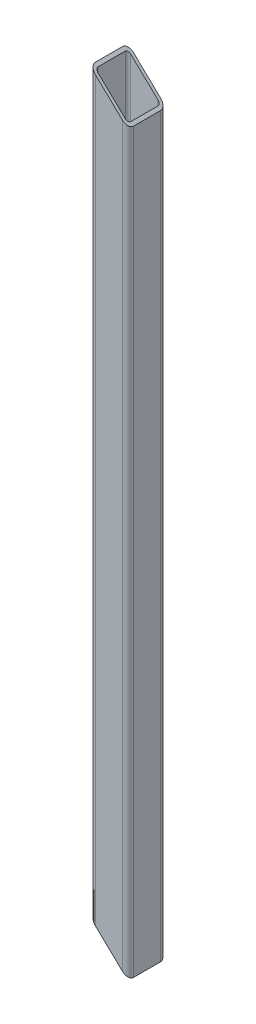
from build123d import *

# Parameters (mm, degrees)
FEATURE_19_WELDMEMBERFEAT_4_MORE_IN_5_DEPTH = 1420.5
CUT_EXTRUDE1_DEPTH                          = 1423.654297431
CUT_EXTRUDE1_DEPTH_BACK                     = 1423.654297431


with BuildPart() as part:
    # Sketch1 → feature 19 (WeldMemberFeat) (+4 more in 5 files) Cold-formed Hollow Structural Square Steel(gb t6728-2002) 70×70×5(1) (new body)
    with BuildSketch(Plane(origin=(0, 0, 0), x_dir=(-1, 0, 0), z_dir=(0, 1, 0))):
        with BuildLine():
            Line((-25, -35), (25, -35))
            ThreePointArc((25, -35), (32.071067812, -32.071067812), (35, -25))
            Line((35, -25), (35, 25))
            ThreePointArc((35, 25), (32.071067812, 32.071067812), (25, 35))
            Line((25, 35), (-25, 35))
            ThreePointArc((-25, 35), (-32.071067812, 32.071067812), (-35, 25))
            Line((-35, 25), (-35, -25))
            ThreePointArc((-35, -25), (-32.071067812, -32.071067812), (-25, -35))
        make_face()
        with BuildLine():
            Line((-25, -30), (25, -30))
            ThreePointArc((25, -30), (28.535533906, -28.535533906), (30, -25))
            Line((30, -25), (30, 25))
            ThreePointArc((30, 25), (28.535533906, 28.535533906), (25, 30))
            Line((25, 30), (-25, 30))
            ThreePointArc((-25, 30), (-28.535533906, 28.535533906), (-30, 25))
            Line((-30, 25), (-30, -25))
            ThreePointArc((-30, -25), (-28.535533906, -28.535533906), (-25, -30))
        make_face(mode=Mode.SUBTRACT)
    extrude(amount=FEATURE_19_WELDMEMBERFEAT_4_MORE_IN_5_DEPTH)

    # 0:feat:20/0 feature 20/0 (ProfileFeature) (+11 more in 7 files) Sketch2 → Cut-Extrude1 (cut, two sides: drawn at the far end of the back side and taken through both)
    with BuildSketch(Plane.XY.offset(35).offset(-CUT_EXTRUDE1_DEPTH_BACK)):
        Polygon((-35, 66.713584391), (35, 0), (-35, 0), align=None)
        Polygon((-35, 1420.5), (35, 1353.786415609), (35, 1420.5), align=None)
    extrude(amount=CUT_EXTRUDE1_DEPTH + CUT_EXTRUDE1_DEPTH_BACK, mode=Mode.SUBTRACT)


solid = part.part
